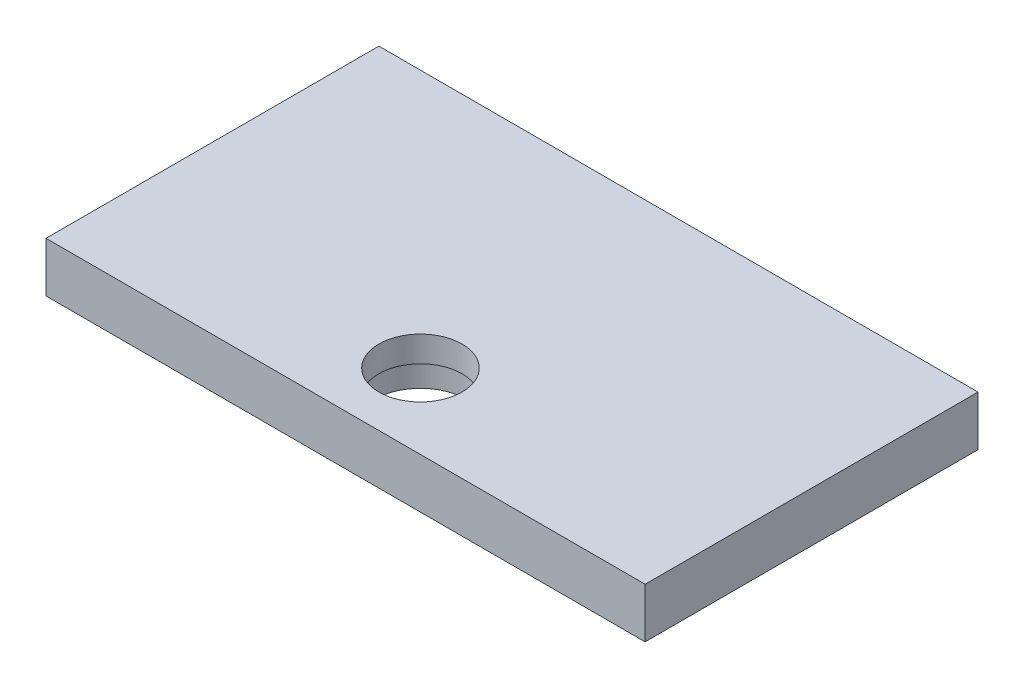
from build123d import *

# Parameters (mm, degrees)
SKETCH_1_W          = 360
SKETCH_1_H          = 200
EXTRUDE_1_DEPTH     = 30
SKETCH_2_R          = 25
CUT_EXTRUDE_1_DEPTH = 209.086520467
SKETCH_3_R          = 27.5
CUT_EXTRUDE_2_DEPTH = 14.53


with BuildPart() as part:
    # 草图1 → 凸台-拉伸1 (new body)
    with BuildSketch(Plane(origin=(0, 0, 0), x_dir=(1, 0, 0), z_dir=(0, 1, 0))):
        Rectangle(SKETCH_1_W, SKETCH_1_H)
    extrude(amount=EXTRUDE_1_DEPTH)

    # 草图2 → 切除-拉伸1 (cut, through all)
    with BuildSketch(Plane.XZ):
        with Locations(Location((0, 55, 0), (0, 0, 270))):
            Circle(SKETCH_2_R)
    extrude(amount=-CUT_EXTRUDE_1_DEPTH, mode=Mode.SUBTRACT)

    # 草图3 → 切除-拉伸2 (cut)
    with BuildSketch(Plane.XZ):
        with Locations(Location((0, 55, 0), (0, 0, 270))):
            Circle(SKETCH_3_R)
    extrude(amount=-CUT_EXTRUDE_2_DEPTH, mode=Mode.SUBTRACT)


solid = part.part
